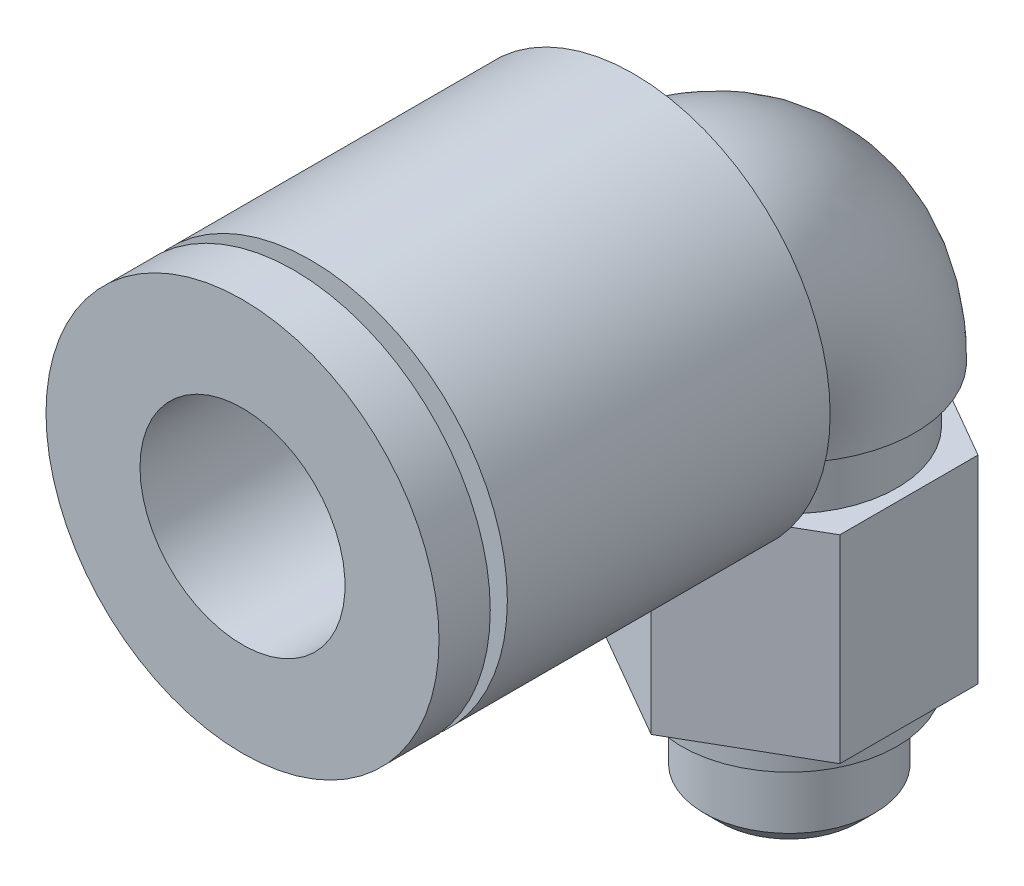
from build123d import *

# Parameters (mm, degrees)
SKETCH_3_R               = 3.67
REVOLVE_2_ANGLE          = 90
EXTRUDE_1_DEPTH          = 5.8
CUT_EXTRUDE_1_DEPTH      = 14
CUT_EXTRUDE_1_DEPTH_BACK = 14
SKETCH_5_R               = 3


with BuildPart() as part:
    # 草图1 → 旋转1 (revolve)
    with BuildSketch(Plane.XY, mode=Mode.PRIVATE) as revolve_1_sk:
        Polygon((0, 0), (-2.01, 0), (-2.5, 0.49), (-2.5, 2.5), (-3.15, 2.5), (-3.15, 10.705), (0, 10.705), align=None)
    revolve(revolve_1_sk.sketch.rotate(Axis((0, 10.705, 0), (0, -1, 0)), 180), axis=Axis((0, 10.705, 0), (0, -1, 0)))

    # 草图3 → 旋转2 (revolve)
    with BuildSketch(Plane(origin=(0, 10.705, 0), x_dir=(1, 0, 0), z_dir=(0, 1, 0))):
        Circle(SKETCH_3_R)
    revolve(axis=Axis((3.68, 10.705, 3.795), (1, 0, 0)), revolution_arc=REVOLVE_2_ANGLE)

    # 草图4 → 凸台-拉伸1 (add)
    with BuildSketch(Plane(origin=(0, 3.25, 0), x_dir=(1, 0, 0), z_dir=(0, 1, 0))):
        Polygon((-3.5, 2.020725942), (-3.5, -2.020725942), (0, -4.041451884), (3.5, -2.020725942), (3.5, 2.020725942), (0, 4.041451884), align=None)
    extrude(amount=EXTRUDE_1_DEPTH)

    # 草图2 → 旋转3 (revolve)
    with BuildSketch(Plane(origin=(0, 14.5, 0), x_dir=(1, 0, 0), z_dir=(0, 1, 0)), mode=Mode.PRIVATE) as revolve_3_sk:
        Polygon((0, -16), (-5.75, -16), (-5.75, -14.5), (-4.5, -14.5), (-4.5, -14), (-5.75, -14), (-5.75, -4.554654828), (-3.68, -4), (-3.68, -3.565), (0, -3.565), align=None)
    revolve(revolve_3_sk.sketch.rotate(Axis((0, 14.5, 3.565), (0, 0, 1)), 180), axis=Axis((0, 14.5, 3.565), (0, 0, 1)))

    # 草图5 → 切除-拉伸1 (cut, two sides: drawn at the far end of the back side and taken through both)
    with BuildSketch(Plane.XY.offset(16).offset(-CUT_EXTRUDE_1_DEPTH_BACK)):
        with Locations(Location((0, 14.5, 0), (0, 0, 180))):
            Circle(SKETCH_5_R)
    extrude(amount=CUT_EXTRUDE_1_DEPTH + CUT_EXTRUDE_1_DEPTH_BACK, mode=Mode.SUBTRACT)


solid = part.part
